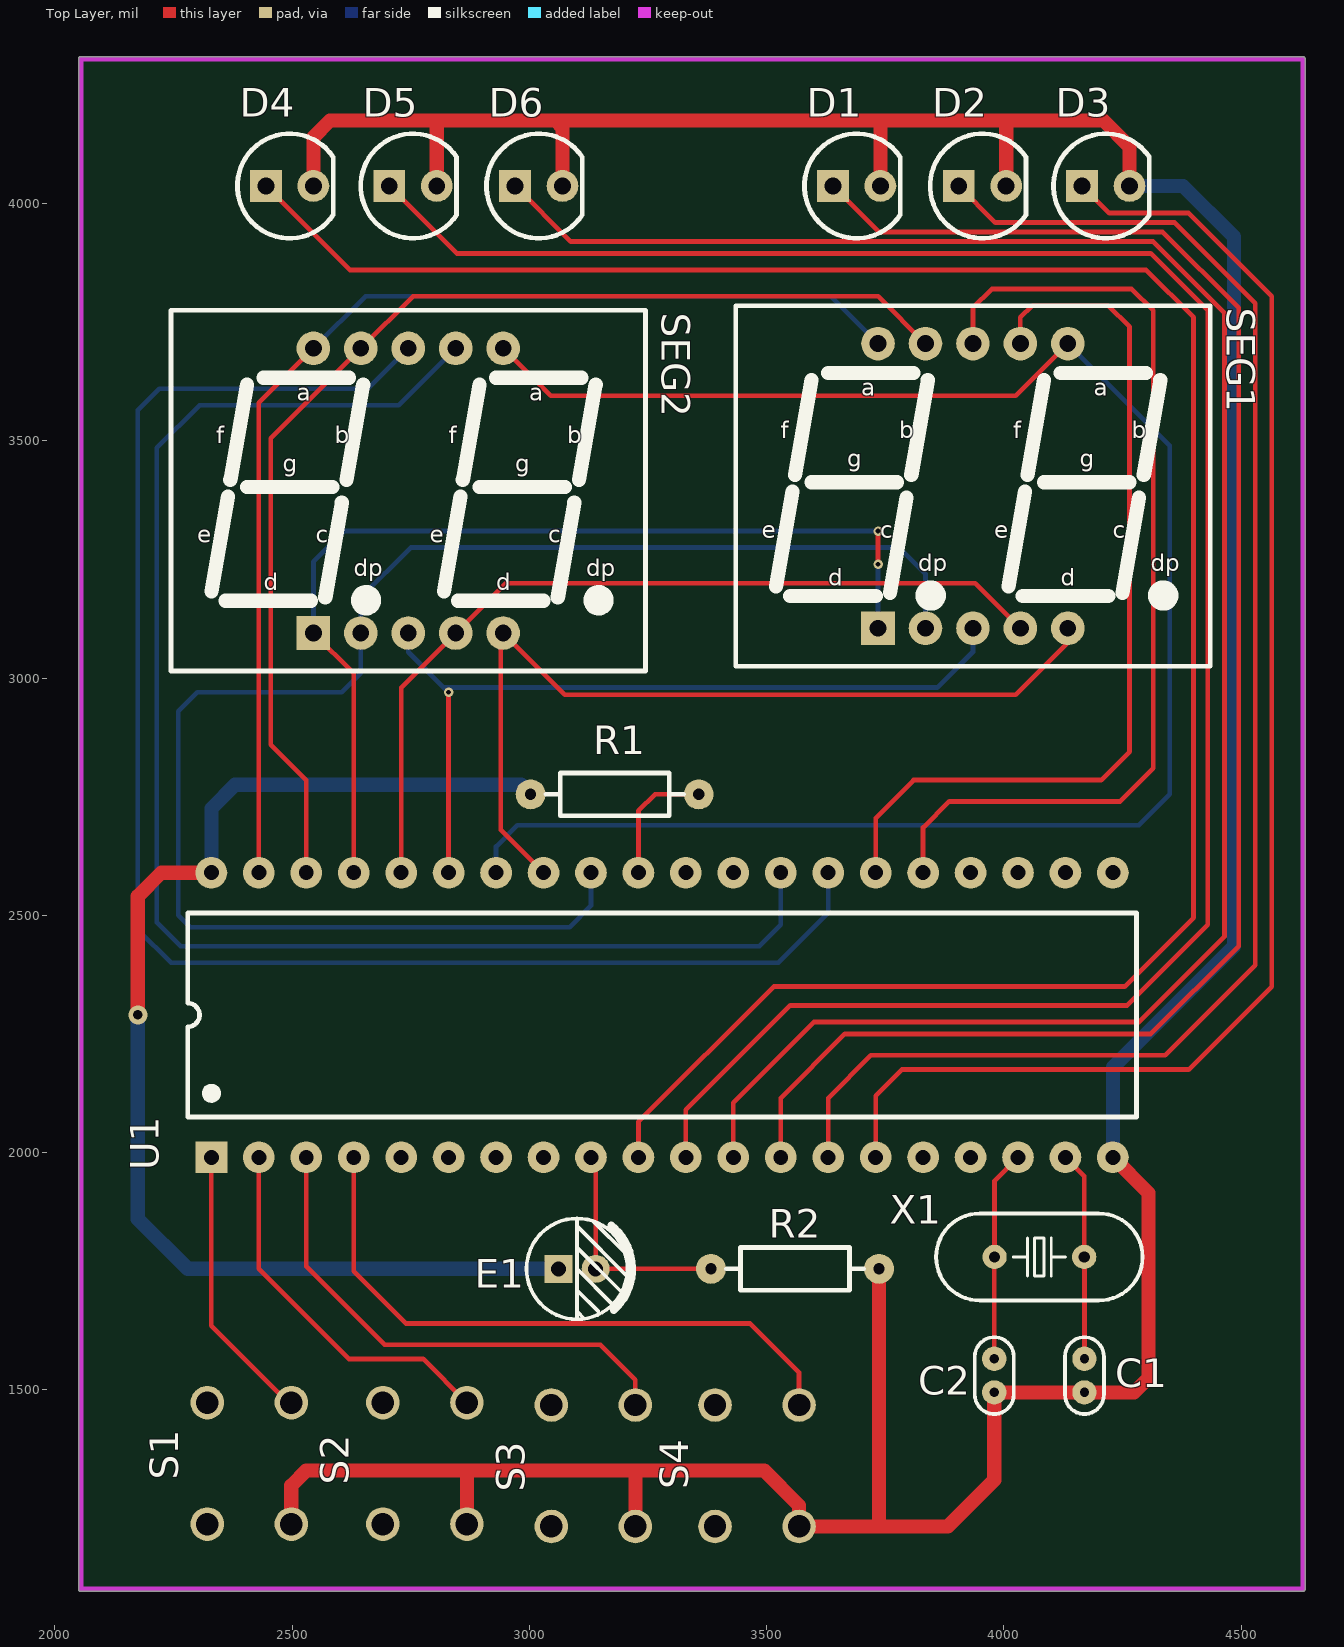
[diagram p0: Top Layer view]
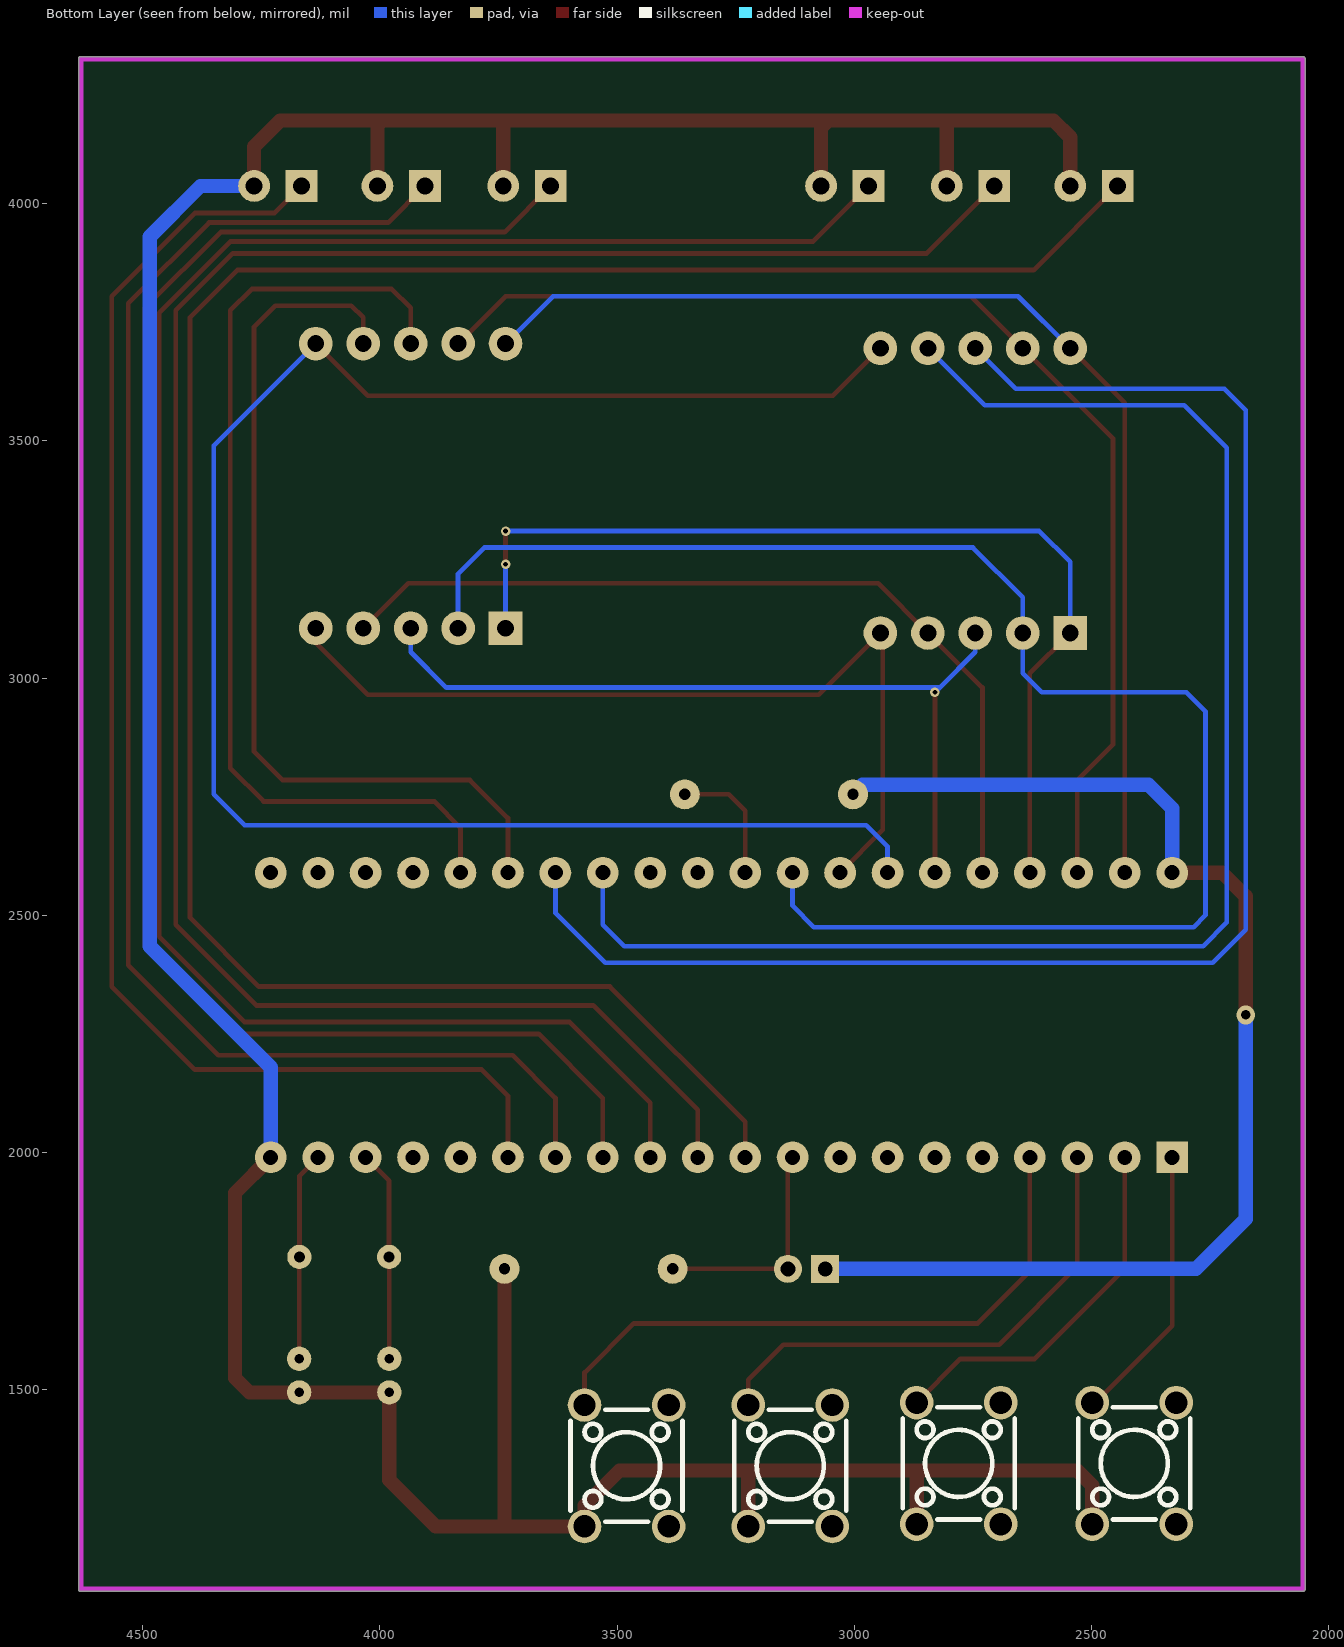
[diagram p1: Bottom Layer view, seen from below]
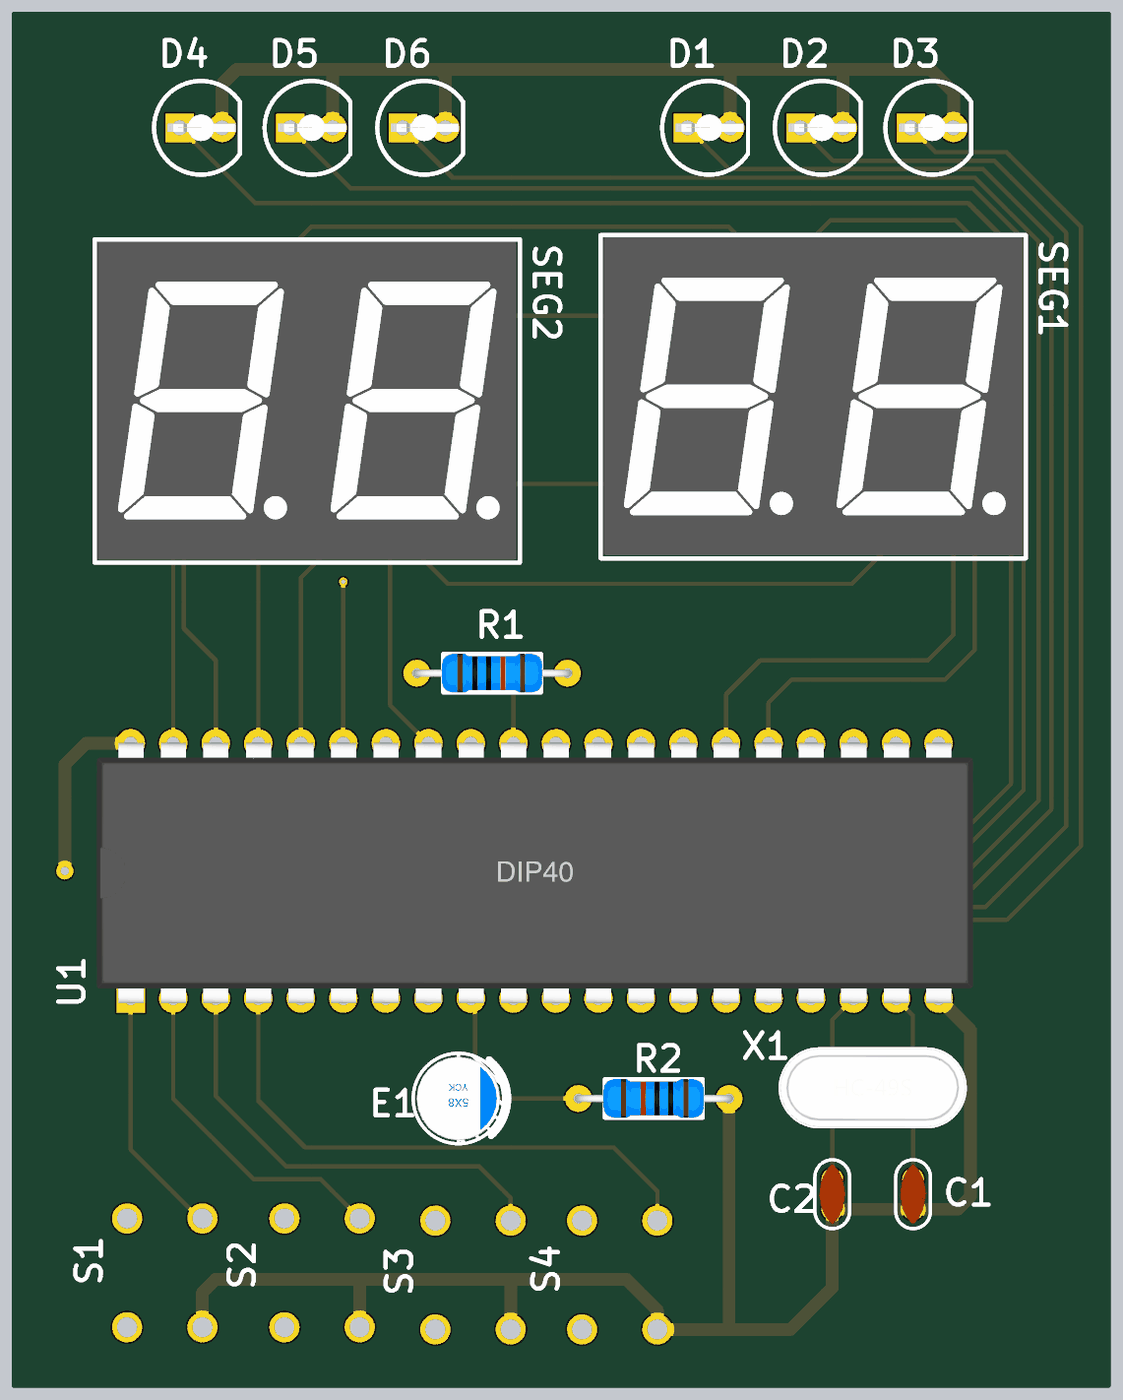
[diagram p2: 3D render of the assembled board from above, using the file's embedded part models]
# Altium PCB MISC84455.PcbDoc
Units mil, origin at the board's own origin, x right, y up, seen from the top; angles counter-clockwise.
Board outline 2585.03 x 3235.03 mil, 2 copper layers (Top Layer, Bottom Layer); 19 components, 28 nets, 100 pads, 4 vias.

## Layer stack, top to bottom (the 12.6 mil dielectric is the usual default, probably not edited)
Top Solder: solder mask 0.4, Solder Resist, Dk 3.5
Top Layer: signal copper 1.4
Dielectric 1: dielectric 12.6, FR-4, Dk 4.8
Bottom Layer: signal copper 1.4
Bottom Solder: solder mask 0.4, Solder Resist, Dk 3.5

## Board outline
2055,1074.98 cw(c2055,1080) 2049.99,1080 2049.99,4305 cw(c2055,4305) 2055,4310.02 4630,4310.02 cw(c4630,4305) 4635.02,4305 4635.02,1080 cw(c4630,1080) 4630,1074.98

## Design rules (kind name [scope] priority, off if disabled: settings)
Clearance [All] p1: gap=10
MinimumSolderMaskSliver [All] p1: minsoldermaskwidth=0
PolygonConnect [All] p1: connectstyle=Relief reliefconductorwidth=10 reliefentries=4 polygonreliefangle="90 Angle" airgapwidth=10
RoutingVias [All] p1: holewidth=28 width=50 viastyle="Through Hole" minholewidth=28 minwidth=50 maxholewidth=28 maxwidth=50
SilkToSilkClearance [All] p1: silktosilkclearance=0
SilkToSolderMaskClearance [IsPad] p1: minsilkscreentomaskgap=0 clearancetoexposedcopper=TRUE
SolderMaskExpansion [All] p1: expansion=4
Width [All] p1: maxlimit=30 minlimit=10 preferedwidth=10
27 further rules are at their usual default settings.

## Components (designator, comment, footprint, x,y, rotation, side; value= is the part's Value field where it differs from the comment)
C1 "30PF" "CC 1.8*3.6" 4170,1530 r90 top
C2 "30PF" "CC 1.8*3.6" 3980,1530 r90 top
D1 "LED" "LED 5MM-W" 3690,4037.17 r0 top
D2 "LED" "LED 5MM-W" 3955,4037.17 r0 top
D3 "LED" "LED 5MM-W" 4215,4037.17 r0 top
D4 "LED" "LED 5MM-W" 2495,4037.17 r0 top
D5 "LED" "LED 5MM-W" 2755,4037.17 r0 top
D6 "LED" "LED 5MM-W" 3020,4037.17 r0 top
E1 "33PF" "CS 2.0*5*8 - C" 3100.63,1755 r180 top
R1 "4.7K" "RS 1/4W" 3180,2755 r0 top
R2 "10K" "RS 1/4W" 3560,1755 r180 top
S1 "Set green" 四脚轻触开关 2410,1345 r270 top
S2 "Set red" 四脚轻触开关 2780,1345 r270 top
S3 "Minus" 四脚轻触开关 3135,1340 r270 top
S4 "Plus" 四脚轻触开关 3480,1340 r270 top
SEG1 "0.56IN-2-K" 0.56IN-2P 3735,3105 r0 top
SEG2 "0.56IN-2-K" 0.56IN-2P 2545,3095 r0 top
U1 "AT89C52" DIP40 3280,2290 r90 top
X1 "12MHz" "OSC HC-49S" 4075,1780 r0 top

## Footprints (in the part's own frame and the unit in brackets; to place one, negate y for a bottom-side part, rotate by r counter-clockwise, add the part's x,y. Pads: shape width x height; smd on the part's side, far side on the other; paste and mask are expansions set on the pad)
0.56IN-2P [mm]
  rect 1.8x1.8 hole 0.9: 1(0,0)
  round 1.8 hole 0.9: 2(2.54,0) 3(5.08,0) 4(7.62,0) 5(10.16,0) 6(10.16,15.24) 7(7.62,15.24) 8(5.08,15.24) 9(2.54,15.24) 10(0,15.24)
  silkscreen extent -7.62,-2.03 17.78,17.27, body extent -7.42,-1.85 17.58,17.14, height 8
"CC 1.8*3.6" [mm] "脚距1.8mm直径3.6mm"
  round 1.3 hole 0.5: 1(-0.9,0) 2(0.9,0)
  silkscreen extent -2.05,-1.04 2.05,1.04, body extent -1.8,-0.8 1.8,0.8, height 3.6
"CS 2.0*5*8 - C" [mm] "脚距2mm , 直径5mm , 高8mm"
  rect 1.5x1.5 hole 0.8: 1(1,0)
  round 1.5 hole 0.8: 2(-1,0)
  silkscreen extent -2.96,-2.7 2.7,2.7, body extent -2.5,-2.5 2.5,2.5, height 8.02
DIP40 [mm]
  rect 1.7x1.7 hole 0.8: 1(-7.62,24.13)
  round 1.7 hole 0.8: 2(-7.62,21.59) 3(-7.62,19.05) 4(-7.62,16.51) 5(-7.62,13.97) 6(-7.62,11.43) 7(-7.62,8.89) 8(-7.62,6.35) 9(-7.62,3.81) 10(-7.62,1.27) 11(-7.62,-1.27) 12(-7.62,-3.81) 13(-7.62,-6.35) 14(-7.62,-8.89) 15(-7.62,-11.43) 16(-7.62,-13.97) 17(-7.62,-16.51) 18(-7.62,-19.05) 19(-7.62,-21.59) 20(-7.62,-24.13) 21(7.62,-24.13) 22(7.62,-21.59) 23(7.62,-19.05) 24(7.62,-16.51) 25(7.62,-13.97) 26(7.62,-11.43) 27(7.62,-8.89) 28(7.62,-6.35) 29(7.62,-3.81) 30(7.62,-1.27) 31(7.62,1.27) 32(7.62,3.81) 33(7.62,6.35) 34(7.62,8.89) 35(7.62,11.43) 36(7.62,13.97) 37(7.62,16.51) 38(7.62,19.05) 39(7.62,21.59) 40(7.62,24.13)
  silkscreen extent -5.46,-25.4 5.46,25.4, body extent -7.91,-26.19 7.65,26.16, height 4.7
"LED 5MM-W" [mm] "白色5mm直插LED"
  rect 1.7x1.7 hole 0.9: 1(-1.27,0)
  round 1.7 hole 0.9: 2(1.27,0)
  silkscreen extent -2.8,-2.8 2.33,2.8, body extent -2.85,-2.85 2.45,2.85, height 8.75
"OSC HC-49S" [mm]
  round 1.3 hole 0.6: 1(-2.4,0) 2(2.4,0)
  silkscreen extent -5.52,-2.32 5.52,2.33, body extent -5.52,-2.32 5.53,2.33, height 4.13
"RS 1/4W" [mm] "直插色环电阻，脚距9mm，直径2.3mm"
  round 1.6 hole 0.6: 1(-4.5,0) 2(4.5,0)
  silkscreen extent -3.68,-1.14 3.68,1.14, body extent -4.72,-1.16 4.73,1.16, height 2.32
四脚轻触开关 [mm]
  round 1.8 hole 1.2 paste+0 mask+0.102: 1(3.25,2.25) 2(-3.25,2.25) 3(3.25,-2.25) 4(-3.25,-2.25)

## Part data
C1 C2: library part CC, "ceramic disc capacitor"
D1 D2 D3 D4 D5 D6: "light-emitting diode"
E1: library part CS, "through-hole solid-state capacitor"
R1 R2: library part R-S, "colour-band resistor"
S1 S2 S3 S4: library part SW-PB, "Switch"
SEG1 SEG2: "2-digit 0.56 inch common-cathode display"
U1: library part STC89C52
X1: library part XTAL-2P, "2-pin passive crystal oscillator"

## Via types
v1: diameter 20, hole 10, Top Layer to Bottom Layer, 3 vias
v2: diameter 40, hole 20, Top Layer to Bottom Layer, 1 vias

## Nets (pads, with @x,y where several pads share a name; then routed paths per layer and width w, separated by ;. In a path a pad name is that pad's centre, name@x,y a point inside that pad or via, vN(x,y) a via of type N, cw(c..) or ccw(c..) an arc to the next point about the centre after c; other vN are vias at no path point)
+5V: E1.1 R1.1 U1.40 | length 2622.3
  Top Layer w30: v2(2175,2290) 2175,2540 2225,2590 U1.40
  Bottom Layer w30: v2(2175,2290) 2175,1860 2280,1755 E1.1 ; U1.40 2330,2725 2380,2775 2982.83,2775 R1.1
A: SEG1.10 SEG2.10 U1.39 | length 2429.6
  Top Layer w10: U1.39 2430,3580 SEG2.10
  Bottom Layer w10: SEG2.10 2655,3805 3635,3805 SEG1.10
B: SEG1.9 SEG2.9 U1.38 | length 2491.8
  Top Layer w10: U1.38 2530,2785 2455,2860 2455,3505 SEG2.9 2755,3805 3735,3805 SEG1.9
C: SEG1.1 SEG2.1 U1.37 | length 2112.1
  Top Layer w10: SEG2.1 2630,3010 U1.37 ; v1(3735,3240) v1(3735,3310)
  Bottom Layer w10: SEG2.1 2545,3245 2610,3310 v1(3735,3310) ; SEG1.1 v1(3735,3240)
D: SEG1.4 SEG2.4 U1.36 | length 1825.5
  Top Layer w10: U1.36 2730,2980 SEG2.4 2950,3200 3940,3200 SEG1.4
E: SEG1.3 SEG2.3 U1.35 | length 1736.3
  Top Layer w10: U1.35 v1(2830,2970)
  Bottom Layer w10: SEG2.3 2745,3055 2820,2980 ; v1(2830,2970) 2820,2980 ; SEG1.3 3935,3055 3860,2980 2820,2980
F: SEG1.6 SEG2.6 U1.34 | length 3836.6
  Top Layer w10: SEG2.6 3045,3595 4025,3595 SEG1.6
  Bottom Layer w10: U1.34 2930,2645 2975,2690 4285,2690 4350,2755 4350,3490 SEG1.6
G: SEG1.5 SEG2.5 U1.33 | length 1863.8
  Top Layer w10: U1.33 2940,2680 2940,3090 SEG2.5 3075,2965 4025,2965 4135,3075 SEG1.5
G1: D6.1 U1.12 | length 4215.6
  Top Layer w10: D6.1 3087.17,3920 4315,3920 4465,3770 4465,2455 4285,2275 3600,2275 3430,2105 U1.12
G2: D3.1 U1.15 | length 3011.4
  Top Layer w10: U1.15 3730,2120 3785,2175 4390,2175 4565,2350 4565,3805 4390,3980 4222.17,3980 D3.1
GND: C1.1 C2.1 D1.2 D2.2 D3.2 D4.2 D5.2 D6.2 R2.1 S1.1 S2.1 S3.1 S4.1 U1.20 | length 8307.6
  Top Layer w30: S1.1 2498.58,1298.58 2530,1330 2870,1330 ; D4.2 2545,4140 2580,4175 2795,4175 ; D5.2 2805,4165 2795,4175 ; S2.1 2868.58,1328.58 2870,1330 ; D6.2 3070,4160 3055,4175 ; S3.1 3223.58,1321.42 3215,1330 ; R2.1 3737.17,1214.88 3740,1212.05 ; D1.2 3740,4175 ; D2.2 4005,4165 3995,4175 ; U1.20 4305,1915 4305,1525 4274.57,1494.57 C1.1 C2.1 3980,1310 3882.05,1212.05 3740,1212.05 ; D3.2 4265,4120 4210,4175 3995,4175 ; 2795,4175 3055,4175 ; 2870,1330 3215,1330 ; 3055,4175 3740,4175 ; 3215,1330 3495,1330 3568.58,1256.42 S4.1 3740,1212.05 ; 3740,4175 3995,4175
  Bottom Layer w30: U1.20 4230,2180 4485,2435 4485,3930 4377.83,4037.17 D3.2
H: SEG1.2 SEG2.2 U1.32 | length 3348.4
  Bottom Layer w10: U1.32 3130,2520 3085,2475 2285,2475 2260,2500 2260,2930 2300,2970 2605,2970 2645,3010 SEG2.2 2645,3170 2750,3275 3780,3275 3835,3220 SEG1.2
NetC1_2: C1.2 U1.19 X1.2 | length 441.1
  Top Layer w10: U1.19 4169.49,1950.51 X1.2 4170,1779.49 C1.2
NetC2_2: C2.2 U1.18 X1.1 | length 445.3
  Top Layer w10: C2.2 3980,1779.49 X1.1 3980.51,1940.51 U1.18
NetE1_2: E1.2 R2.2 U1.9 | length 482
  Top Layer w10: U1.9 3140,1980 E1.2 R2.2
NetR1_2: R1.2 U1.31 | length 271.7
  Top Layer w10: U1.31 3230,2720 3265,2755 R1.2
NetS1_2: S1.2 U1.1 | length 590.7
  Top Layer w10: U1.1 2330,1635 2492.05,1472.95 S1.2
NetS2_2: S2.2 U1.2 | length 790.4
  Top Layer w10: U1.2 2430,1755 2620,1565 2776.54,1565 S2.2
NetS3_2: S3.2 U1.3 | length 1075.9
  Top Layer w10: U1.3 2530,1760 2695,1595 3150,1595 3223.58,1521.42 S3.2
NetS4_2: S4.2 U1.4 | length 1335.5
  Top Layer w10: U1.4 2630,1750 2740,1640 3465,1640 3568.58,1536.42 S4.2
R1: D4.1 U1.10 | length 4757.9
  Top Layer w10: D4.1 2622.17,3860 4300,3860 4400,3760 4400,2495 4255,2350 3515,2350 3230,2065 U1.10
R2: D1.1 U1.13 | length 3529.1
  Top Layer w10: U1.13 3530,2115 3665,2250 4310,2250 4495,2435 4495,3780 4335,3940 3737.17,3940 D1.1
S1: SEG2.7 U1.28 | length 3181.3
  Bottom Layer w10: SEG2.7 2725,3575 2305,3575 2215,3485 2215,2485 2265,2435 3485,2435 3530,2480 U1.28
S2: SEG2.8 U1.27 | length 3331.3
  Bottom Layer w10: SEG2.8 2660,3610 2220,3610 2175,3565 2175,2470 2245,2400 3525,2400 3630,2505 U1.27
S3: SEG1.7 U1.26 | length 1917
  Top Layer w10: U1.26 3730,2705 3810,2785 4205,2785 4265,2845 4265,3740 4220,3785 4060,3785 4035,3760 SEG1.7
S4: SEG1.8 U1.25 | length 2087
  Top Layer w10: U1.25 3830,2685 3885,2740 4245,2740 4315,2810 4315,3775 4270,3820 3975,3820 3935,3780 SEG1.8
Y1: D5.1 U1.11 | length 4490.1
  Top Layer w10: D5.1 2847.17,3895 4310,3895 4430,3775 4430,2480 4260,2310 3550,2310 3330,2090 U1.11
Y2: D2.1 U1.14 | length 3263.4
  Top Layer w10: U1.14 3630,2115 3720,2205 4340,2205 4530,2395 4530,3790 4360,3960 3982.17,3960 D2.1
pads on no net: S1.3 S1.4 S2.3 S2.4 S3.3 S3.4 S4.3 S4.4 U1.5 U1.6 U1.7 U1.8 U1.16 U1.17 U1.21 U1.22 U1.23 U1.24 U1.29 U1.30

## Keep-outs
Keep-Out Layer:
  lines w10: 2055,1080 4630,1080 4630,4305 2055,4305 2055,1080